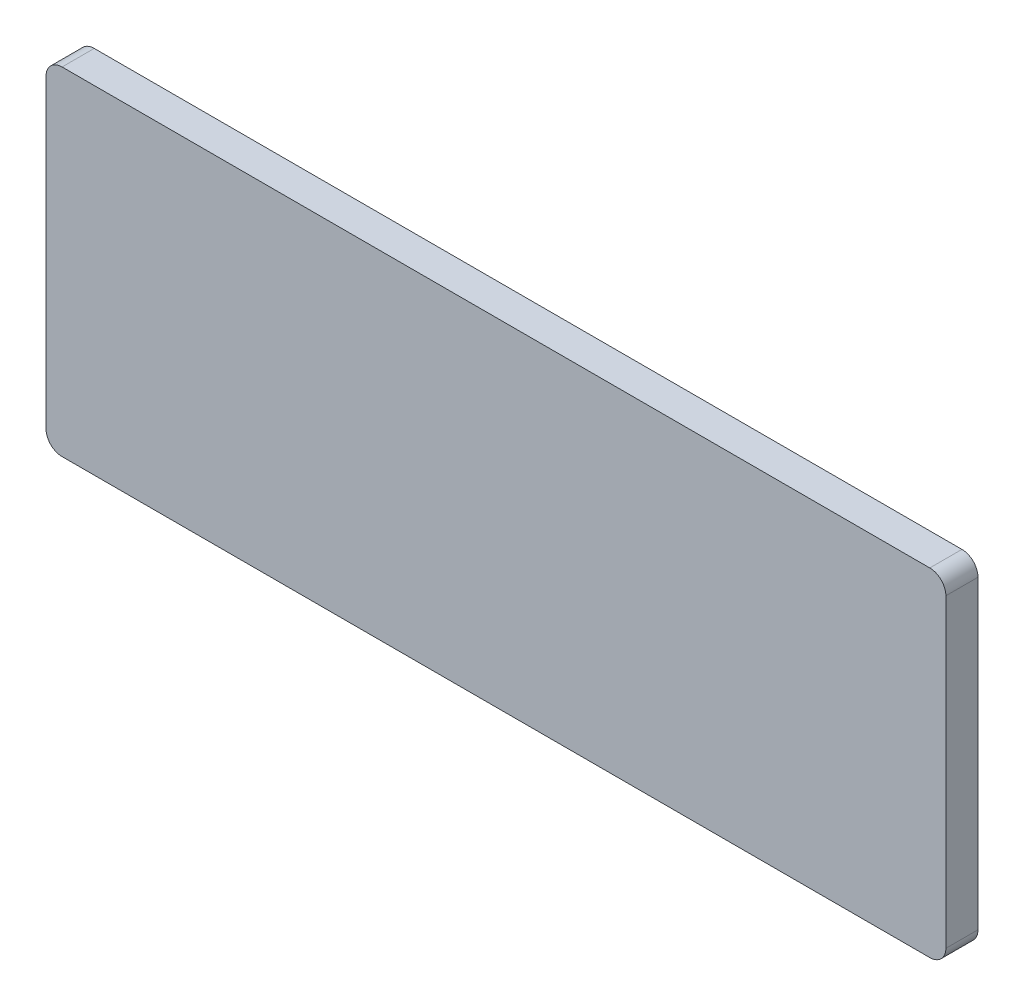
from build123d import *

# Parameters (mm, degrees)
BOSS_EXTRUDE1_DEPTH = 4


with BuildPart() as part:
    # Sketch1 → Boss-Extrude1 (new body)
    with BuildSketch(Plane.XY):
        with BuildLine():
            Line((54, 21), (-54, 21))
            ThreePointArc((-54, 21), (-55.414213562, 20.414213562), (-56, 19))
            Line((-56, 19), (-56, -19))
            ThreePointArc((-56, -19), (-55.414213562, -20.414213562), (-54, -21))
            Line((-54, -21), (54, -21))
            ThreePointArc((54, -21), (55.414213562, -20.414213562), (56, -19))
            Line((56, -19), (56, 19))
            ThreePointArc((56, 19), (55.414213562, 20.414213562), (54, 21))
        make_face()
    extrude(amount=BOSS_EXTRUDE1_DEPTH)


solid = part.part
